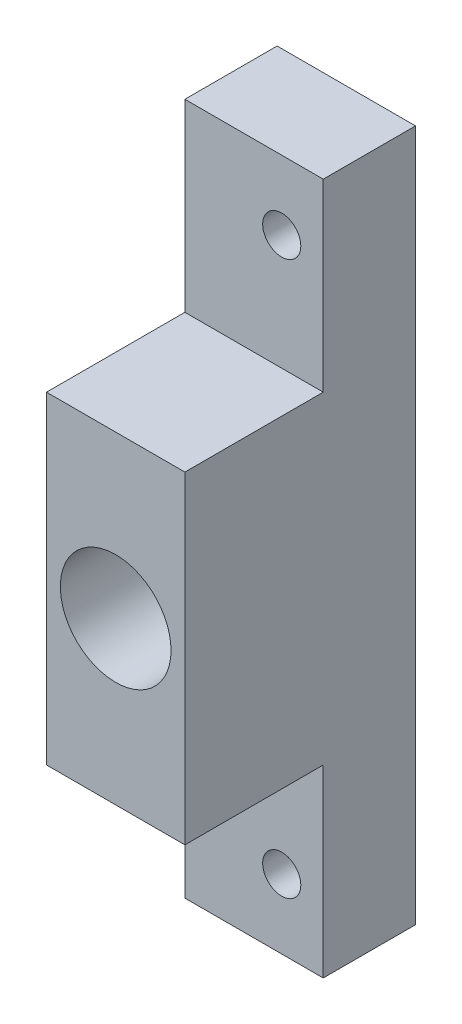
SolidWorks part; units mm, degrees
ref_plane "Front Plane" through (0, 0, 0) normal (0, 0, 1) x (1, 0, 0)
ref_plane "Top Plane" through (0, 0, 0) normal (0, 1, 0) x (1, 0, 0)
ref_plane "Right Plane" through (0, 0, 0) normal (1, 0, 0) x (0, 0, -1)
other "Configuration Table"
sketch "Sketch1" plane through (0, 0, 0) normal (0, 0, 1) x (1, 0, 0)
  line L2 (-32, 37.5) -> (-12.5, 37.5) construction
  line L3 (-22, 37.5) -> (-22, -37.5)
  line L4 (-22, -37.5) -> (-37, -37.5)
  line L5 (-12.5, -37.5) -> (-32, -37.5) construction
  line L7 (-22, -26.25) -> (-22, 22.5) construction
  line L8 (-37, -37.5) -> (-37, 37.5)
  line L9 (-37, 37.5) -> (-22, 37.5)
  dimension "D1" = 0
extrude "Boss-Extrude1" add sketch "Sketch1" along normal blind 25
sketch "Sketch2" plane through (0, 0, 25) normal (0, 0, 1) x (1, 0, 0)
  circle A0 centre (-26.5, 30) radius 2.067
  circle A1 centre (-26.5, -30) radius 2.067
extrude "Cut-Extrude1" cut sketch "Sketch2" against normal blind 25
sketch "Sketch3" plane through (0, 0, 25) normal (0, 0, 1) x (1, 0, 0)
  line L0 (-37, 37.5) -> (-22, 37.5)
  line L1 (-22, 37.5) -> (-22, 17.5)
  line L2 (-22, -37.5) -> (-22, 37.5) construction
  line L3 (-22, 17.5) -> (-37, 17.5)
  line L4 (-37, 37.5) -> (-37, -37.5) construction
  line L5 (-37, 17.5) -> (-37, 37.5)
  line L6 (-22, 0) -> (-37, 0) construction
  line L7 (-22, -17.5) -> (-37, -17.5)
  line L8 (-22, -37.5) -> (-22, -17.5)
  line L9 (-37, -37.5) -> (-22, -37.5)
  line L10 (-37, -17.5) -> (-37, -37.5)
extrude "Cut-Extrude2" cut sketch "Sketch3" against normal blind 15
sketch "Sketch4" plane through (0, 0, 25) normal (0, 0, 1) x (1, 0, 0)
  line L0 (-22, 0) -> (-37, 0) construction
  line L1 (-22, -17.5) -> (-22, 17.5) construction
  line L2 (-37, 17.5) -> (-37, -17.5) construction
  circle A0 centre (-29.5, 0) radius 6
  dimension "D1" = 12
extrude "Cut-Extrude3" cut sketch "Sketch4" against normal blind 20
